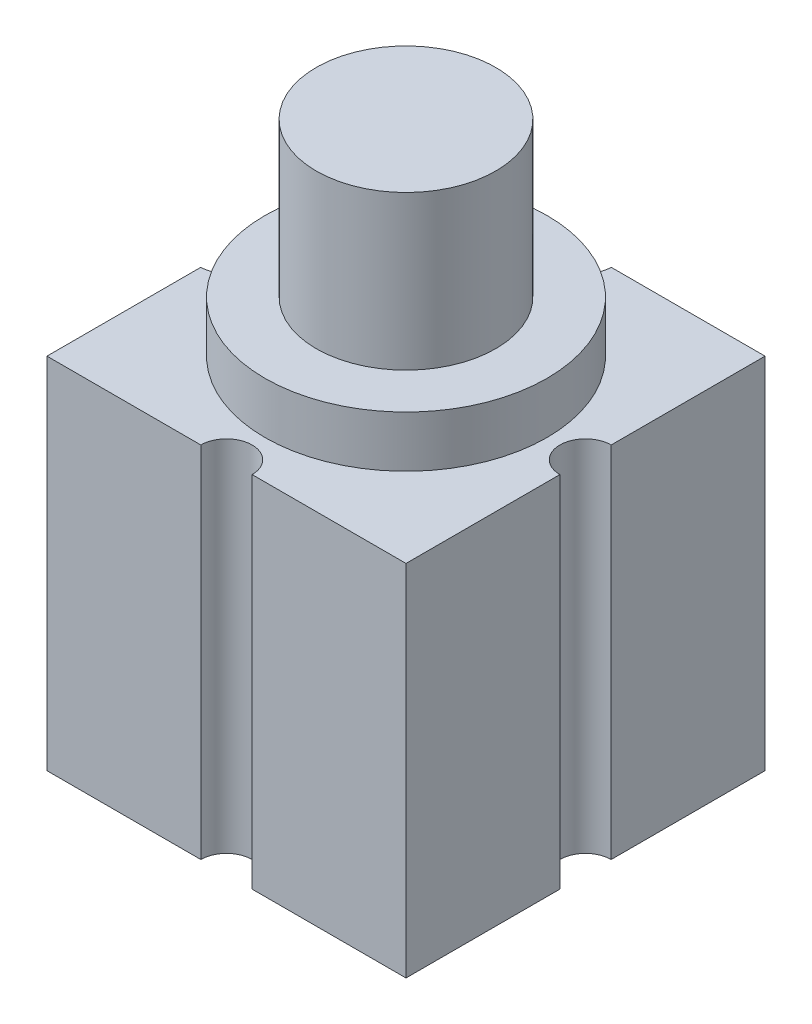
SolidWorks part; units mm, degrees
ref_plane "Front Plane" through (0, 0, 0) normal (0, 0, 1) x (1, 0, 0)
ref_plane "Top Plane" through (0, 0, 0) normal (0, 1, 0) x (1, 0, 0)
ref_plane "Right Plane" through (0, 0, 0) normal (1, 0, 0) x (0, 0, -1)
sketch "Sketch1" plane through (0, 0, 0) normal (0, 1, 0) x (1, 0, 0)
  line L0 (5, 35) -> (35, 35)
  line L1 (-35, -35) -> (-5, -35)
  line L2 (-35, -35) -> (-35, -5)
  line L3 (-35, 35) -> (-5, 35)
  line L4 (35, -35) -> (35, -5)
  line L5 (-35, -35) -> (35, 35) construction
  line L6 (-35, 35) -> (35, -35) construction
  line L7 (-35, 5) -> (-35, 35)
  line L8 (35, 5) -> (35, 35)
  line L9 (5, -35) -> (35, -35)
  arc A0 (-5, 35) -> (5, 35) centre (0, 35) ccw
  arc A1 (35, 5) -> (35, -5) centre (35, 0) ccw
  arc A2 (5, -35) -> (-5, -35) centre (0, -35) ccw
  arc A3 (-35, -5) -> (-35, 5) centre (-35, 0) ccw
  point P0 (0, 0)
  dimension "D3" = 10
  dimension "D4" = 10
  dimension "D5" = 10
  dimension "D6" = 10
  dimension "D1" = 70
  dimension "D2" = 70
extrude "Boss-Extrude1" add sketch "Sketch1" along normal blind 70
sketch "Sketch2" plane through (0, 0, 0) normal (0, -1, 0) x (1, 0, 0)
  circle A0 centre (0, 0) radius 20
  dimension "D1" = 40
extrude "Cut-Extrude1" cut sketch "Sketch2" against normal blind 10
sketch "Sketch3" plane through (0, 70, 0) normal (0, 1, 0) x (1, 0, 0)
  circle A0 centre (0, 0) radius 27.5
  dimension "D1" = 55
extrude "Boss-Extrude2" add sketch "Sketch3" along normal blind 10
sketch "Sketch4" plane through (0, 80, 0) normal (0, 1, 0) x (1, 0, 0)
  circle A0 centre (0, 0) radius 17.5
  dimension "D1" = 35
extrude "Boss-Extrude3" add sketch "Sketch4" along normal blind 30
